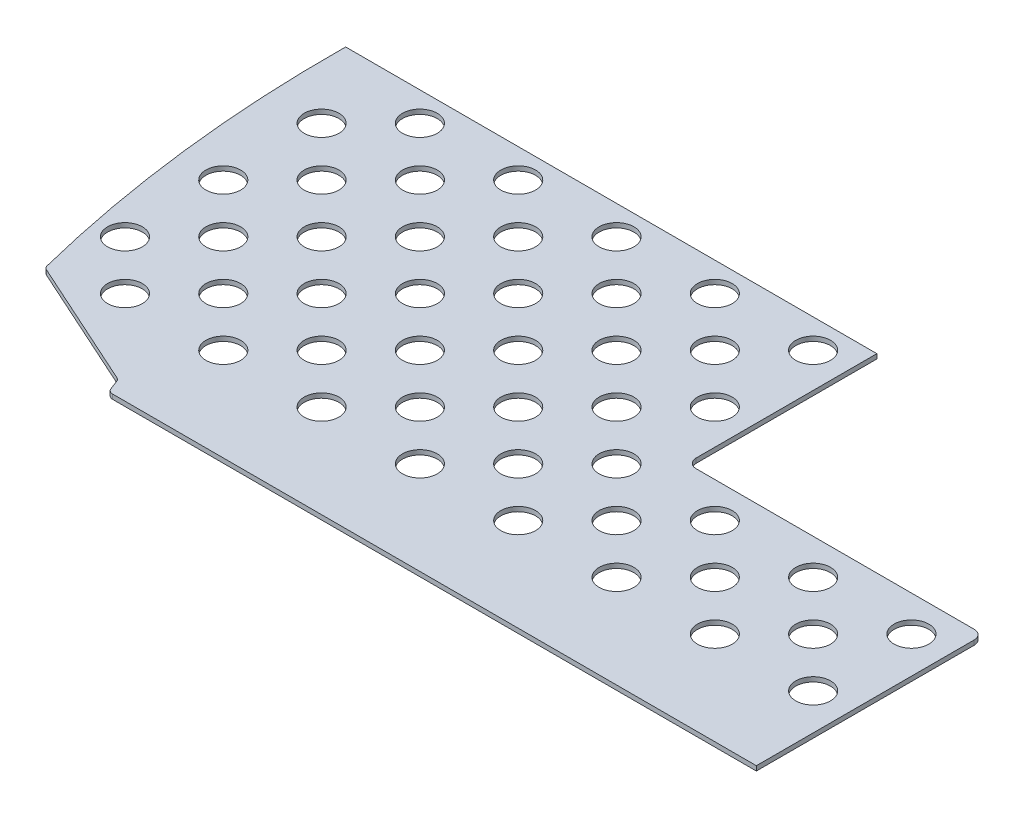
SolidWorks part; units mm, degrees
material "Q235"
ref_plane "Front Plane" through (0, 0, 0) normal (0, 0, 1) x (1, 0, 0)
ref_plane "Top Plane" through (0, 0, 0) normal (0, 1, 0) x (1, 0, 0)
ref_plane "Right Plane" through (0, 0, 0) normal (1, 0, 0) x (0, 0, -1)
ref_plane "Plane1" through (0, 0, 0) normal (0, -1, 0) x (1, 0, 0)
sketch "Sketch1" plane through (0, 0, 0) normal (0, -1, 0) x (1, 0, 0)
  line L0 (119.6346, -7.2267) -> (116.5775, -15.2864)
  line L1 (113.9643, -18.0682) -> (3.0077, -68.2917)
  line L2 (-34.5249, -364) -> (423.9751, -364)
  line L3 (423.9751, -364) -> (423.9751, -208)
  line L4 (431.9751, -200) -> (671.9751, -200)
  line L5 (679.9751, -192) -> (679.9751, -4)
  line L6 (679.9751, -4) -> (124.3096, -4)
  arc A0 (116.5775, -15.2864) -> (113.9643, -18.0682) centre (111.9025, -13.5131) cw
  arc A1 (3.0077, -68.2917) -> (0.2207, -71.6265) centre (5.0695, -72.8468) ccw
  arc A2 (0.2207, -71.6265) -> (-34.5249, -364) centre (1116.4179, -352.5266) ccw
  arc A3 (423.9751, -208) -> (431.9751, -200) centre (431.9751, -208) cw
  arc A4 (671.9751, -200) -> (679.9751, -192) centre (671.9751, -192) ccw
  arc A5 (124.3096, -4) -> (119.6346, -7.2267) centre (124.3096, -9) ccw
  circle A6 centre (393.9751, -254.1472) radius 15
  circle A7 centre (351.5487, -296.5736) radius 15
  circle A8 centre (309.1223, -339) radius 15
  circle A9 centre (393.9751, -169.2944) radius 15
  circle A10 centre (351.5487, -211.7208) radius 15
  circle A11 centre (309.1223, -254.1472) radius 15
  circle A12 centre (266.6959, -296.5736) radius 15
  circle A13 centre (224.2694, -339) radius 15
  circle A14 centre (478.8279, -169.2944) radius 15
  circle A15 centre (436.4015, -126.868) radius 15
  circle A16 centre (393.9751, -84.4416) radius 15
  circle A17 centre (351.5487, -126.868) radius 15
  circle A18 centre (309.1223, -169.2944) radius 15
  circle A19 centre (266.6959, -211.7208) radius 15
  circle A20 centre (224.2694, -254.1472) radius 15
  circle A21 centre (181.843, -296.5736) radius 15
  circle A22 centre (139.4166, -339) radius 15
  circle A23 centre (563.6807, -169.2944) radius 15
  circle A24 centre (521.2543, -126.868) radius 15
  circle A25 centre (478.8279, -84.4416) radius 15
  circle A26 centre (309.1223, -84.4416) radius 15
  circle A27 centre (266.6959, -126.868) radius 15
  circle A28 centre (224.2694, -169.2944) radius 15
  circle A29 centre (181.843, -211.7208) radius 15
  circle A30 centre (139.4166, -254.1472) radius 15
  circle A31 centre (96.9902, -296.5736) radius 15
  circle A32 centre (54.5638, -339) radius 15
  circle A33 centre (648.5335, -169.2944) radius 15
  circle A34 centre (606.1071, -126.868) radius 15
  circle A35 centre (563.6807, -84.4416) radius 15
  circle A36 centre (224.2694, -84.4416) radius 15
  circle A37 centre (181.843, -126.868) radius 15
  circle A38 centre (139.4166, -169.2944) radius 15
  circle A39 centre (96.9902, -211.7208) radius 15
  circle A40 centre (54.5638, -254.1472) radius 15
  circle A41 centre (12.1374, -296.5736) radius 15
  circle A42 centre (648.5335, -84.4416) radius 15
  circle A43 centre (139.4166, -84.4416) radius 15
  circle A44 centre (96.9902, -126.868) radius 15
  circle A45 centre (54.5638, -169.2944) radius 15
  circle A46 centre (12.1374, -211.7208) radius 15
  circle A47 centre (54.5638, -84.4416) radius 15
  circle A48 centre (12.1374, -126.868) radius 15
  circle A49 centre (393.9751, -339) radius 15
  dimension "D3" = 714.5
  dimension "D6" = 1151
  dimension "D8" = 30
  dimension "D47" = 5
  dimension "D48" = 5
  dimension "D50" = 8
  dimension "D51" = 8
  dimension "D52" = 5
  dimension "D1" = 196
  dimension "D2" = 256
  dimension "D79" = 360
other "Align group 1"
other "Align group 2"
extrude "Boss-Extrude1" add sketch "Sketch1" against normal blind 4
